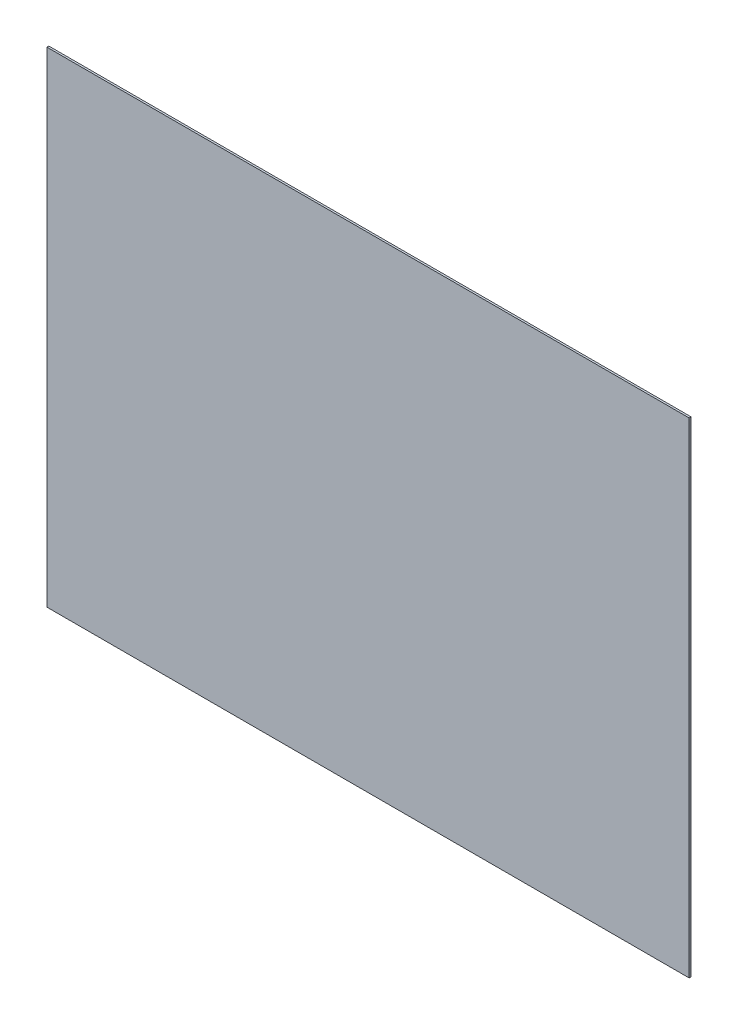
from build123d import *

# Parameters (mm, degrees)
SKETCH1_W           = 1000
SKETCH1_H           = 755
BOSS_EXTRUDE1_DEPTH = 3


with BuildPart() as part:
    # Sketch1 → Boss-Extrude1 (new body)
    with BuildSketch(Plane.XY):
        with Locations((500, 377.5)):
            Rectangle(SKETCH1_W, SKETCH1_H)
    extrude(amount=BOSS_EXTRUDE1_DEPTH)


solid = part.part
